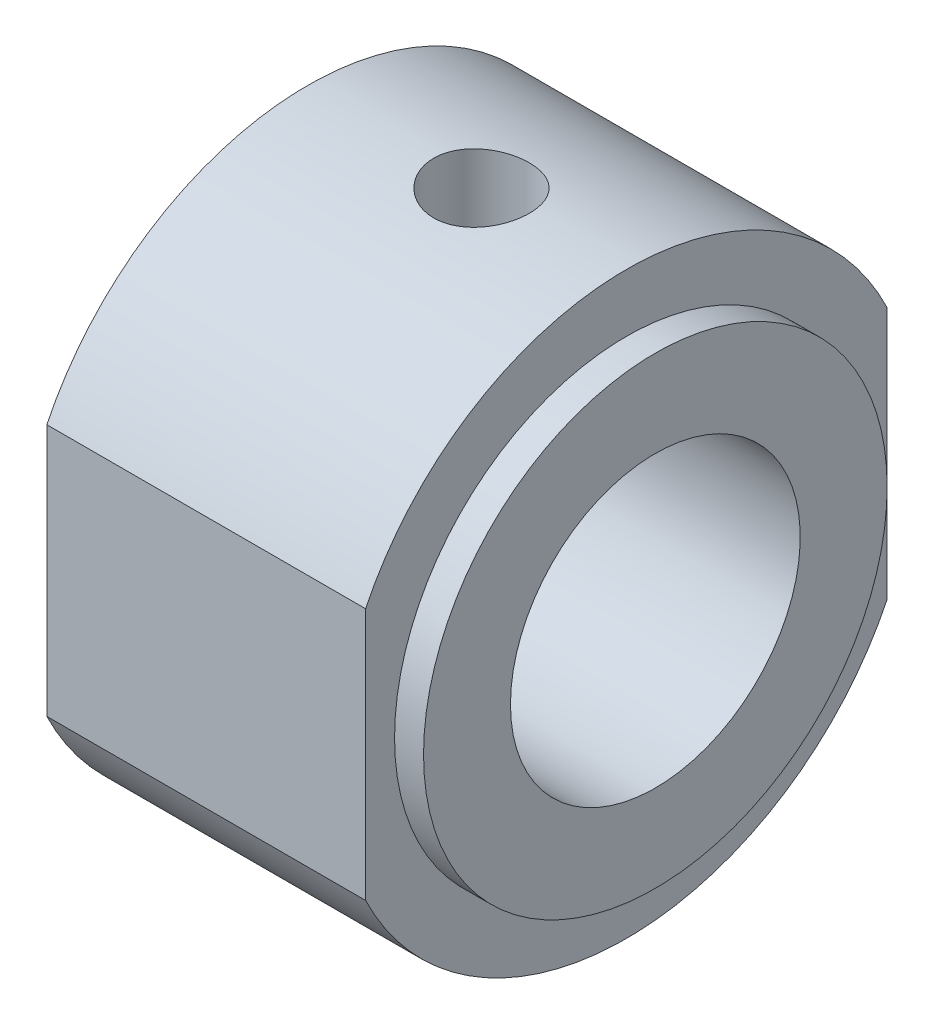
from build123d import *

# Parameters (mm, degrees)
SKETCH2_OUTSIDE_W      = 28.144
SKETCH2_OUTSIDE_H      = 28.144
SKETCH2_OUTSIDE_W_2    = 18
SKETCH2_OUTSIDE_H_2    = 25
CUT_EXTRUDE1_DEPTH     = 19.547236991
M4_TAPPED_HOLE1_REACH  = 27
M4_TAPPED_HOLE1_BORE_R = 1.65


with BuildPart() as part:
    # Sketch1 → Revolve1 (revolve)
    with BuildSketch(Plane.XY, mode=Mode.PRIVATE) as revolve1_sk:
        Polygon((0, 5), (0, 10), (11, 10), (11, 8), (12, 8), (12, 5), align=None)
    revolve(revolve1_sk.sketch.rotate(Axis((0, 0, 0), (1, 0, 0)), 90), axis=Axis((0, 0, 0), (1, 0, 0)))

    # Sketch2 outside → Cut-Extrude1 (cut, through all)
    with BuildSketch(Plane.ZY):
        Rectangle(SKETCH2_OUTSIDE_W, SKETCH2_OUTSIDE_H)
        Rectangle(SKETCH2_OUTSIDE_W_2, SKETCH2_OUTSIDE_H_2, mode=Mode.SUBTRACT)
    extrude(amount=-CUT_EXTRUDE1_DEPTH, mode=Mode.SUBTRACT)

    # M4 Tapped Hole1 bore → M4 Tapped Hole1 (cut, up to next)
    with BuildSketch(Plane(origin=(0, 10, 0), x_dir=(-1, 0, 0), z_dir=(0, 1, 0)), mode=Mode.PRIVATE) as m4_tapped_hole1_sk1:
        with Locations((-6, 0)):
            Circle(M4_TAPPED_HOLE1_BORE_R)
    m4_tapped_hole1_tool1 = extrude(m4_tapped_hole1_sk1.sketch, amount=-M4_TAPPED_HOLE1_REACH, mode=Mode.PRIVATE) & part.part
    add(m4_tapped_hole1_tool1.solids().sort_by_distance((6, 10, 0))[0], mode=Mode.SUBTRACT)


solid = part.part
